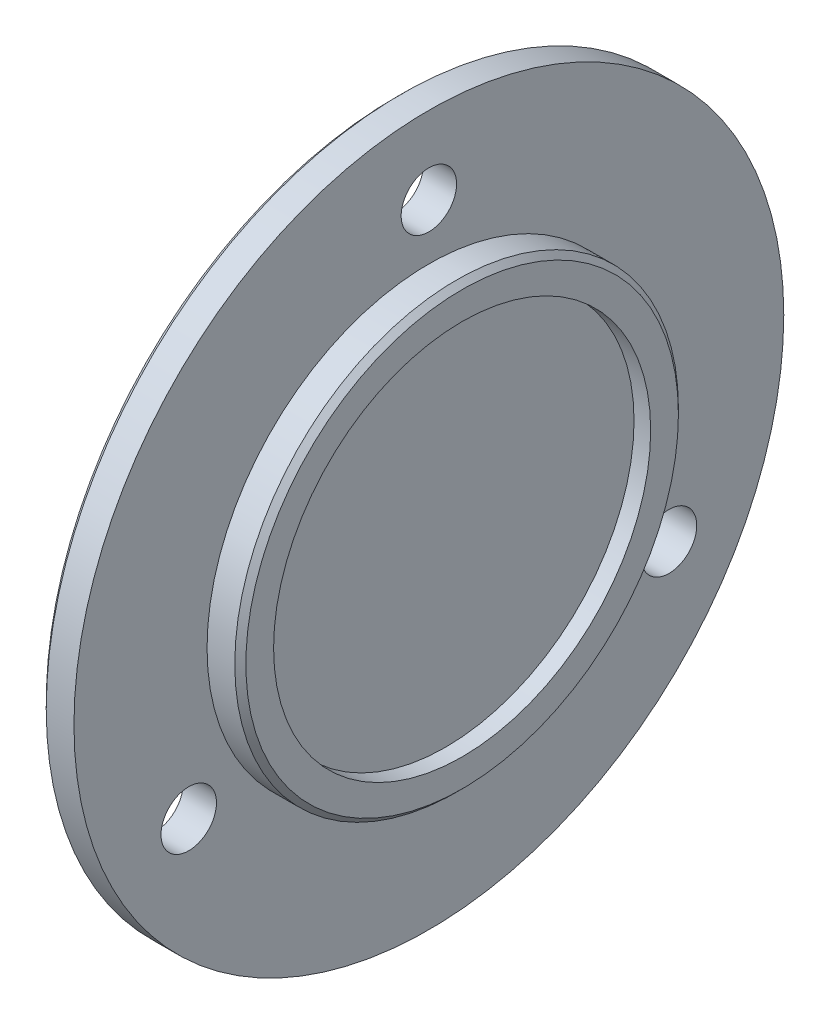
from build123d import *

# Parameters (mm, degrees)
SKETCH1_R           = 32
BOSS_EXTRUDE1_DEPTH = 3
SKETCH2_R           = 20
BOSS_EXTRUDE2_DEPTH = 3
SKETCH3_R           = 17
CUT_EXTRUDE1_DEPTH  = 1.5
SKETCH4_R           = 2.5
CUT_EXTRUDE2_DEPTH  = 36.5
CHAMFER1_SIZE       = 0.5


with BuildPart() as part:
    # Sketch1 → Boss-Extrude1 (new body)
    with BuildSketch(Plane(origin=(0, 0, 0), x_dir=(0, 0, -1), z_dir=(1, 0, 0))):
        Circle(SKETCH1_R)
    extrude(amount=BOSS_EXTRUDE1_DEPTH)

    # Sketch2 → Boss-Extrude2 (add)
    with BuildSketch(Plane(origin=(3, 0, 0), x_dir=(0, 0, -1), z_dir=(1, 0, 0))):
        Circle(SKETCH2_R)
    extrude(amount=BOSS_EXTRUDE2_DEPTH)

    # Sketch3 → Cut-Extrude1 (cut)
    with BuildSketch(Plane(origin=(6, 0, 0), x_dir=(0, 0, -1), z_dir=(1, 0, 0))):
        Circle(SKETCH3_R)
    extrude(amount=-CUT_EXTRUDE1_DEPTH, mode=Mode.SUBTRACT)

    # Sketch4 → Cut-Extrude2 (cut)
    with BuildSketch(Plane.ZY):
        with Locations((0, 25)):
            Circle(SKETCH4_R)
        with Locations((21.650635095, -12.5)):
            Circle(SKETCH4_R)
        with Locations((-21.650635095, -12.5)):
            Circle(SKETCH4_R)
    extrude(amount=-CUT_EXTRUDE2_DEPTH, mode=Mode.SUBTRACT)

    # Chamfer1
    chamfer1_edges = [part.edges().sort_by_distance(p)[0] for p in [
        (0, 0, 32),
        (6, 0, 20),
    ]]
    chamfer(chamfer1_edges, length=CHAMFER1_SIZE)


solid = part.part
